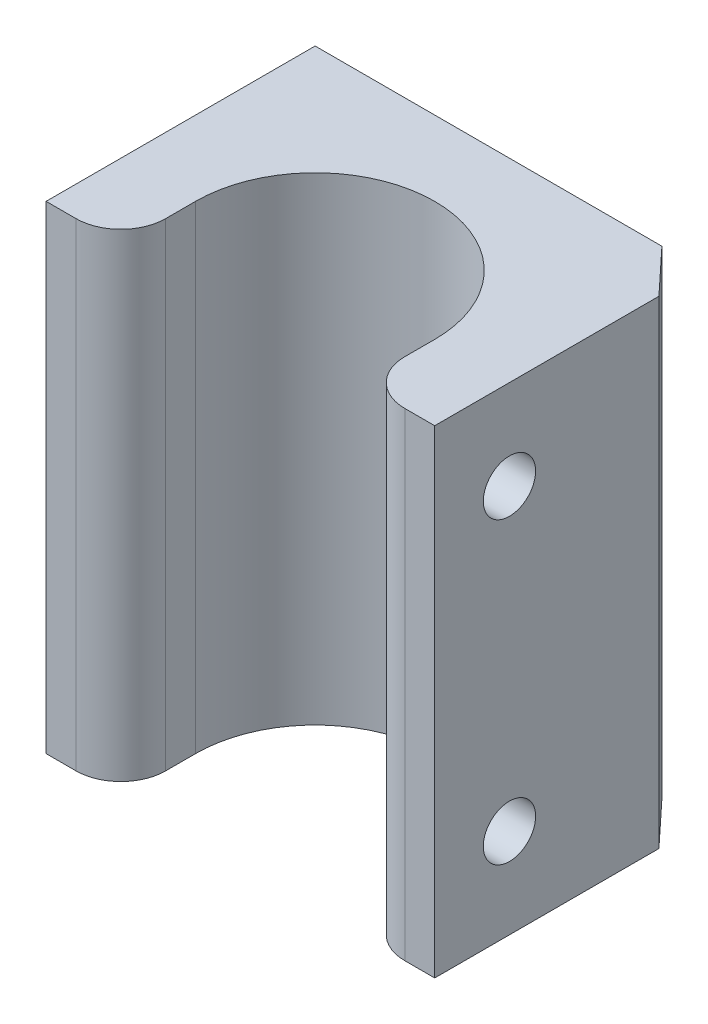
SolidWorks part; units mm, degrees
ref_plane "Front Plane" through (0, 0, 0) normal (0, 0, 1) x (1, 0, 0)
ref_plane "Top Plane" through (0, 0, 0) normal (0, 1, 0) x (1, 0, 0)
ref_plane "Right Plane" through (0, 0, 0) normal (1, 0, 0) x (0, 0, -1)
sketch "Sketch1" plane through (0, 0, 0) normal (0, 1, 0) x (1, 0, 0)
  line L0 (-8, -10) -> (-8, -12)
  line L1 (-13, -15) -> (-11, -15)
  line L2 (-13, -15) -> (-13, 15)
  line L5 (-13, -15) -> (10.5641, 12.1893) construction
  line L6 (-13, 15) -> (13, -15) construction
  line L7 (8, -10) -> (8, -12)
  line L8 (11, -15) -> (13, -15)
  line L9 (13, -15) -> (13, 0)
  line L15 (-13, 15) -> (-1, 15)
  line L19 (13, 0) -> (-1, 15)
  arc A0 (8, -10) -> (-8, -10) centre (0, -10) ccw
  arc A1 (8, -12) -> (11, -15) centre (11, -12) ccw
  arc A2 (-8, -12) -> (-11, -15) centre (-11, -12) cw
  point P0 (0, 0)
  point P15 (8, -15)
  point P18 (-8, -15)
  dimension "D1" = 16
  dimension "D9" = 3
  dimension "D2" = 30
  dimension "D3" = 5
  dimension "D4" = 15
  dimension "D5" = 0
  dimension "D6" = 5
  dimension "D7" = 5
  dimension "D8" = 12
extrude "Boss-Extrude1" add sketch "Sketch1" along normal blind 32
sketch "Sketch2" plane through (13, 0, 0) normal (1, 0, 0) x (0, 0, -1)
  line L0 (-15, 32) -> (-15, 0) construction
  line L1 (-15, 32) -> (0, 32) construction
  circle A0 centre (-10, 26) radius 1.75
  circle A1 centre (-10, 6) radius 1.75
  dimension "D1" = 3.5
  dimension "D2" = 3.5
  dimension "D3" = 20
  dimension "D4" = 5
  dimension "D5" = 5
  dimension "D6" = 6
extrude "Cut-Extrude1" cut sketch "Sketch2" against normal blind 10
sketch "Sketch3" plane through (0, 32, 0) normal (0, 1, 0) x (1, 0, 0)
  line L0 (-1, 15) -> (-13, 15) construction
  line L1 (-42.9739, 28.663) -> (24.4235, 28.663)
  line L2 (-42.9739, 28.663) -> (-42.9739, 3)
  line L3 (-42.9739, 3) -> (24.4235, 3)
  line L4 (24.4235, 28.663) -> (24.4235, 3)
  dimension "D1" = 12
extrude "Cut-Extrude2" cut sketch "Sketch3" against normal through all
sketch "Sketch4" plane through (-13, 0, 0) normal (-1, 0, 0) x (0, 0, 1)
  line L0 (-3, 32) -> (15, 32) construction
  line L1 (-3, 32) -> (-3, 0) construction
  circle A0 centre (0, 6) radius 1.75
  circle A1 centre (0, 26) radius 1.75
  dimension "D1" = 3.5
  dimension "D2" = 3.5
  dimension "D3" = 20
  dimension "D4" = 6
  dimension "D5" = 3
  dimension "D6" = 3
extrude "Cut-Extrude3" cut sketch "Sketch4" against normal blind 10
